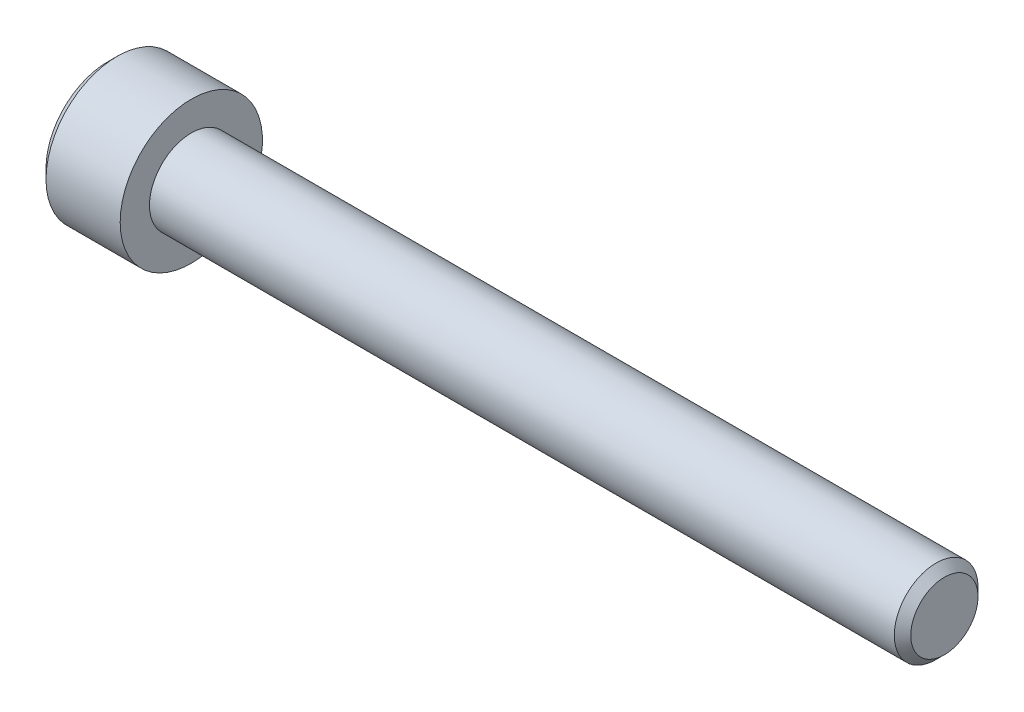
SolidWorks part; units mm, degrees
ref_plane "Front Plane" through (0, 0, 0) normal (0, 0, 1) x (1, 0, 0)
ref_plane "Top Plane" through (0, 0, 0) normal (0, 1, 0) x (1, 0, 0)
ref_plane "Right Plane" through (0, 0, 0) normal (1, 0, 0) x (0, 0, -1)
sketch "Sketch1" plane through (0, 0, 0) normal (0, 0, 1) x (1, 0, 0)
  line L0 (-5, 0) -> (-5, 3.6833)
  line L1 (-5, 3.6833) -> (-4.4333, 4.25)
  line L2 (-4.4333, 4.25) -> (0, 4.25)
  line L3 (0, 4.25) -> (0, 2.5)
  line L4 (0, 2.5) -> (44.5085, 2.5)
  line L5 (44.5085, 2.5) -> (45, 2.0085)
  line L6 (45, 2.0085) -> (45, 0)
  line L7 (45, 0) -> (-5, 0)
  line L8 (45, 0) -> (-5, 0) construction
revolve "Revolve1" add sketch "Sketch1" angle 360 about L8
cosmetic thread "Cosmetic Thread1" parameters "D1"=44.1488, "D2"=4.0171
sketch "Sketch2" plane through (0, 0, 0) normal (0, 0, 1) x (1, 0, 0)
  line L0 (-5, 0) -> (-5, 2)
  line L1 (-5, 2) -> (-2.5, 2)
  line L2 (-2.5, 2) -> (-1.9641, 0)
  line L3 (-1.9641, 0) -> (-5, 0)
  line L4 (-1.9641, 0) -> (-5, 0) construction
revolve "Cut-Revolve1" cut sketch "Sketch2" angle 360 about L4
ref_plane "Plane1" through (-5, 0, 0) normal (1, 0, 0) x (0, 0, -1)
sketch "Sketch3" plane through (-5, 0, 0) normal (1, 0, 0) x (0, 0, -1)
  line L0 (-2, 1.1547) -> (-2, -1.1547)
  line L1 (-2, -1.1547) -> (0, -2.3094)
  line L2 (0, -2.3094) -> (2, -1.1547)
  line L3 (2, -1.1547) -> (2, 1.1547)
  line L4 (2, 1.1547) -> (0, 2.3094)
  line L5 (0, 2.3094) -> (-2, 1.1547)
extrude "Cut-Extrude1" cut sketch "Sketch3" along normal blind 2.5
